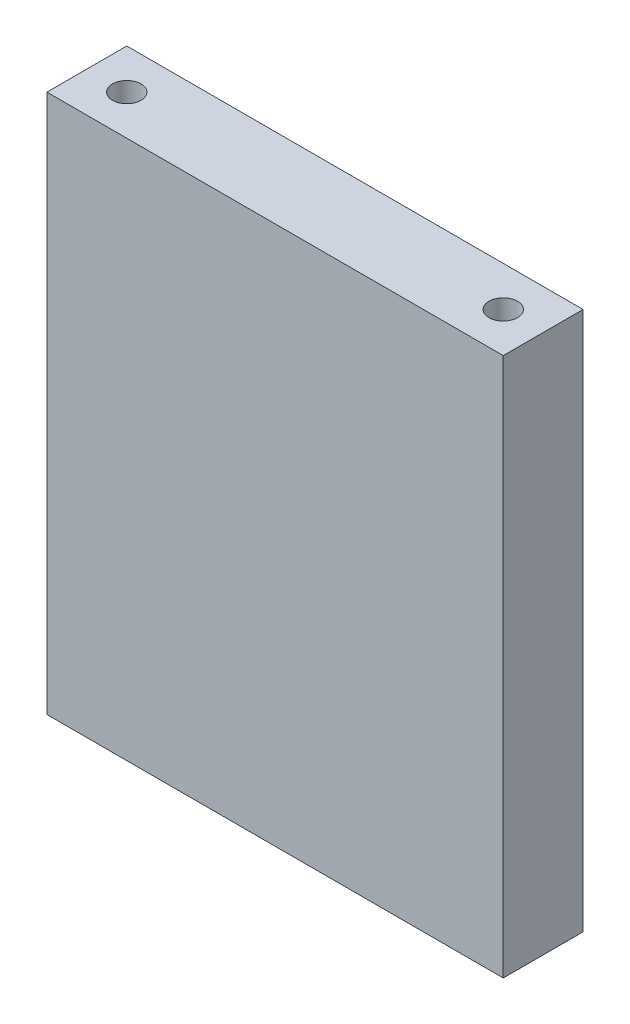
SolidWorks part; units mm, degrees
ref_plane "前视" through (0, 0, 0) normal (0, 0, 1) x (1, 0, 0)
ref_plane "上视" through (0, 0, 0) normal (0, 1, 0) x (1, 0, 0)
ref_plane "右视" through (0, 0, 0) normal (1, 0, 0) x (0, 0, -1)
sketch "草图1" plane through (0, 0, 0) normal (0, 0, 1) x (1, 0, 0)
  line L1 (-40, 47.25) -> (40, 47.25)
  line L2 (-40, 47.25) -> (-40, -47.25)
  line L3 (-40, -47.25) -> (40, -47.25)
  line L4 (40, 47.25) -> (40, -47.25)
  line L5 (-40, 47.25) -> (40, -47.25) construction
  line L6 (-40, -47.25) -> (40, 47.25) construction
  point P0 (0, 0)
  dimension "D1" = 80
  dimension "D2" = 94.5
extrude "凸台-拉伸1" add sketch "草图1" along normal blind 14
hole_wizard "M6 螺纹孔1" positions "草图3" profile "草图2" tap size "M6" standard "GB"
sketch "草图3" plane through (0, -47.25, 0) normal (0, -1, 0) x (-1, 0, 0)
  point P0 (-21, -7)
  point P3 (21, -7)
sketch "草图2" plane through (21, -47.25, 7) normal (1, 0, 0) x (0, 0, -1)
  line L0 (0, 0) -> (0, 18.5022)
  line L1 (0, 18.5022) -> (2.5, 17)
  line L2 (2.5, 17) -> (2.5, 0)
  line L5 (2.5, 0) -> (0, 0)
  line L10 (0, 18.5022) -> (-2.5, 17) construction
  line L11 (0, -6.35) -> (0, 107.95) construction
  dimension "螺纹孔钻头直径" = 5
  dimension "螺纹孔钻头深度" = 17
  dimension "导头角度" = 118
cosmetic thread "孔螺蚊线1" parameters "D1"=12, "D2"=6
cosmetic thread "孔螺蚊线2" parameters "D1"=12, "D2"=6
hole_wizard "M6 螺纹孔2" positions "草图5" profile "草图4" tap size "M6" standard "GB"
sketch "草图5" plane through (0, 47.25, 0) normal (0, 1, 0) x (1, 0, 0)
  point P0 (33, -7)
  point P2 (-33, -7)
sketch "草图4" plane through (33, 47.25, 7) normal (1, 0, 0) x (0, 0, 1)
  line L0 (0, 0) -> (0, 18.5022)
  line L1 (0, 18.5022) -> (2.5, 17)
  line L2 (2.5, 17) -> (2.5, 0)
  line L5 (2.5, 0) -> (0, 0)
  line L10 (0, 18.5022) -> (-2.5, 17) construction
  line L11 (0, -6.35) -> (0, 107.95) construction
  dimension "螺纹孔钻头直径" = 5
  dimension "螺纹孔钻头深度" = 17
  dimension "导头角度" = 118
cosmetic thread "孔螺蚊线3" parameters "D1"=12, "D2"=6
cosmetic thread "孔螺蚊线4" parameters "D1"=12, "D2"=6
